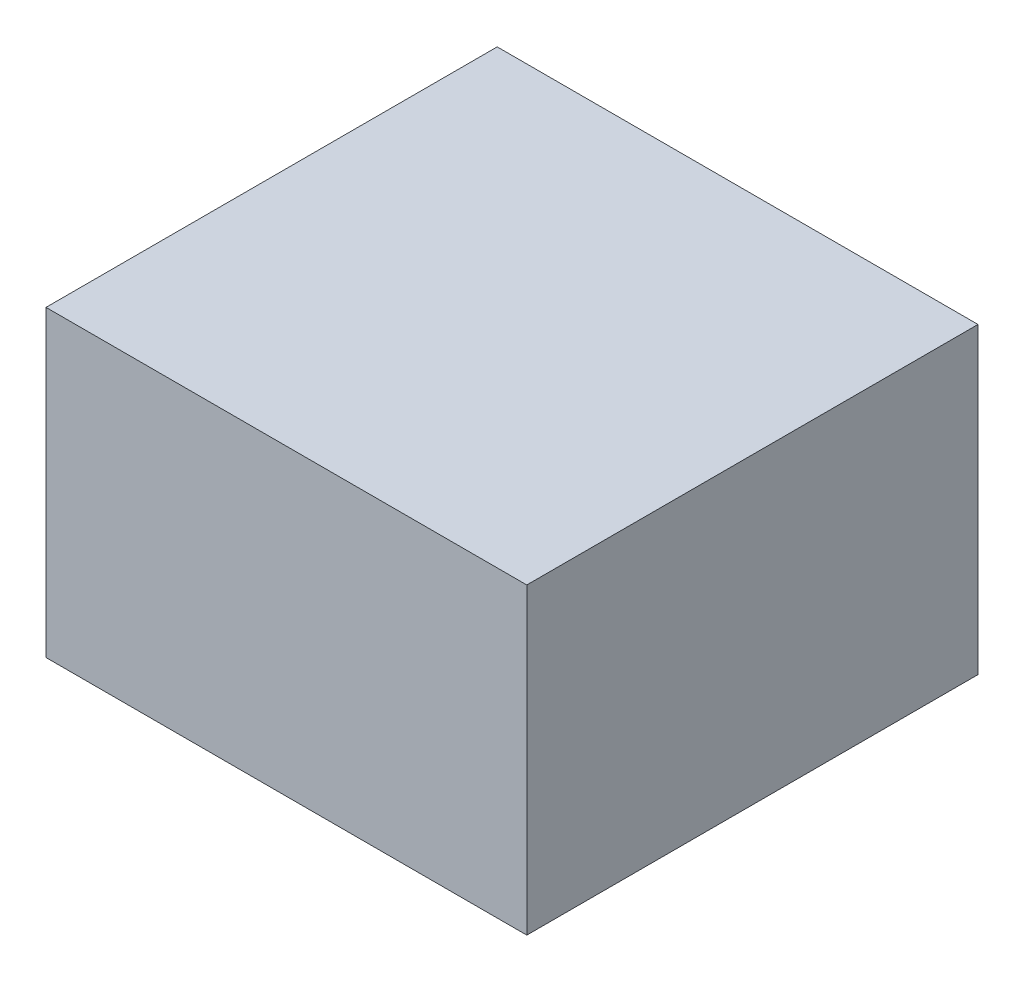
from build123d import *

# Parameters (mm, degrees)
SKETCH1_W           = 6.5
SKETCH1_H           = 6.1
BOSS_EXTRUDE1_DEPTH = 4.1


with BuildPart() as part:
    # Sketch1 → Boss-Extrude1 (new body)
    with BuildSketch(Plane(origin=(0, 0, 0), x_dir=(1, 0, 0), z_dir=(0, 1, 0))):
        with Locations((3.25, 3.05)):
            Rectangle(SKETCH1_W, SKETCH1_H)
    extrude(amount=BOSS_EXTRUDE1_DEPTH)


solid = part.part
